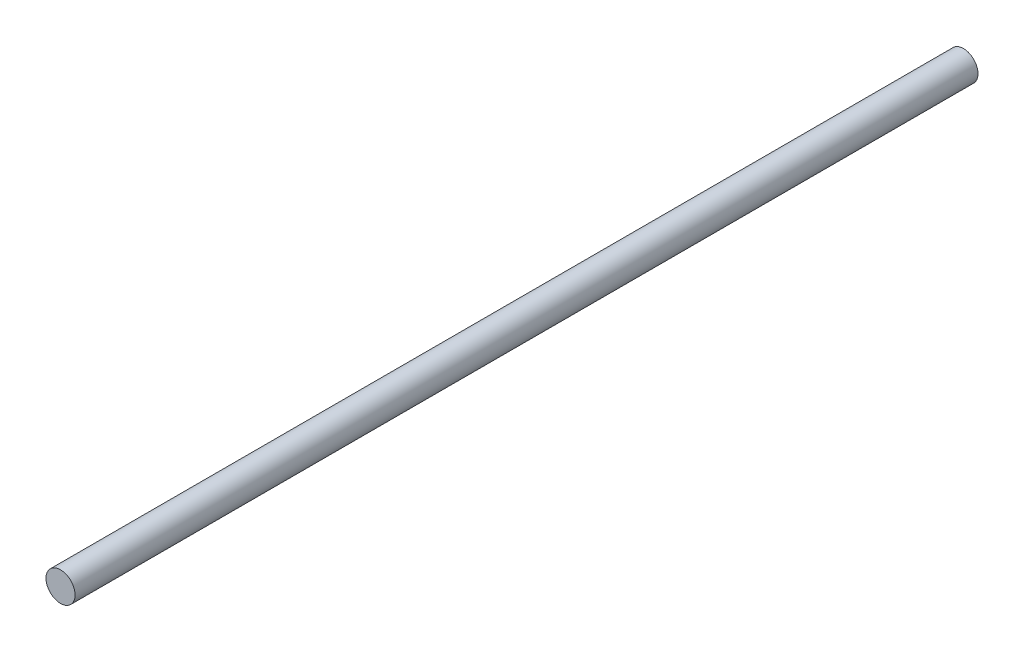
SolidWorks part; units mm, degrees
ref_plane "Front Plane" through (0, 0, 0) normal (0, 0, 1) x (1, 0, 0)
ref_plane "Top Plane" through (0, 0, 0) normal (0, 1, 0) x (1, 0, 0)
ref_plane "Right Plane" through (0, 0, 0) normal (1, 0, 0) x (0, 0, -1)
sketch "Sketch1" plane through (0, 0, 0) normal (0, 0, 1) x (1, 0, 0)
  circle A0 centre (0, 0) radius 2
  dimension "D1" = 4
extrude "Boss-Extrude1" add sketch "Sketch1" along normal mid plane 124
